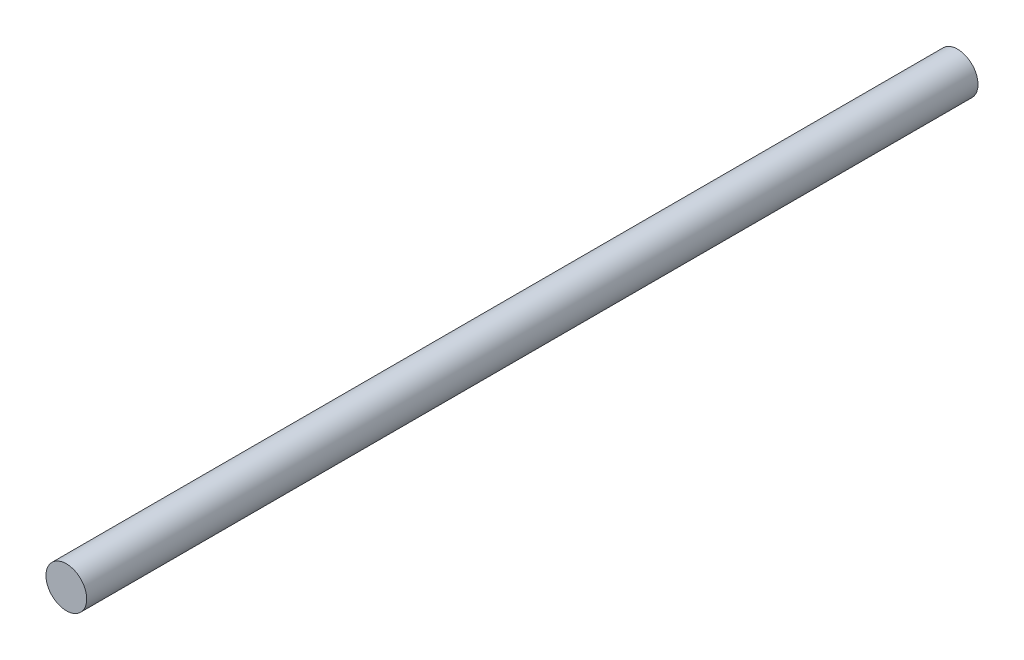
from build123d import *

# Parameters (mm, degrees)
SKETCH_1_R      = 8
EXTRUDE_1_DEPTH = 350


with BuildPart() as part:
    # 草图1 → 凸台-拉伸1 (new body)
    with BuildSketch(Plane.XY):
        Circle(SKETCH_1_R)
    extrude(amount=EXTRUDE_1_DEPTH)


solid = part.part
